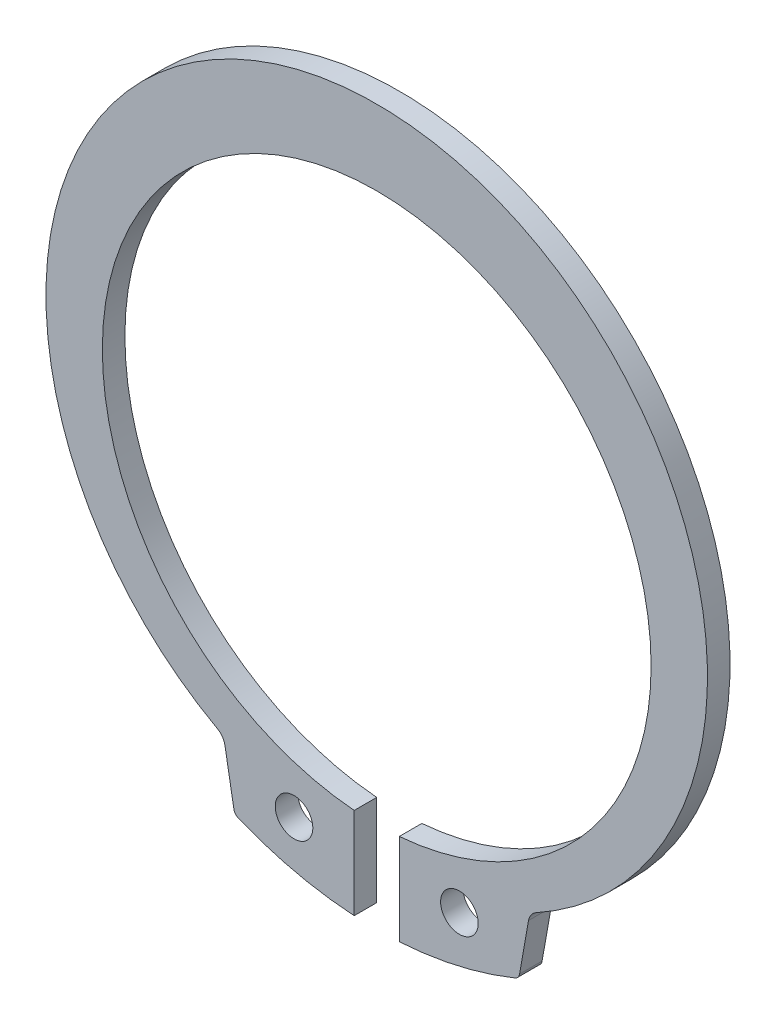
from build123d import *

# Parameters (mm, degrees)
EXTRUDE_972_DEPTH      = 0.75
EXTRUDE_972_DEPTH_BACK = 0.75
SKETCH_1_R             = 1.25


with BuildPart() as part:
    # 草图1 → Extrude 972 (new, two sides: drawn at the far end of the back side and taken through both)
    with BuildSketch(Plane.XY.offset(-EXTRUDE_972_DEPTH_BACK)):
        with BuildLine():
            Line((-1.5, -19.438251703), (-1.5, -25.503659518))
            ThreePointArc((-1.5, -25.503659518), (-5.420429348, -24.937738298), (-9.196831336, -23.742405238))
            ThreePointArc((-9.196831336, -23.742405238), (-9.396824452, -23.593447727), (-9.5, -23.366422634))
            Line((-9.5, -23.366422634), (-10.097014043, -19.980587746))
            ThreePointArc((-10.097014043, -19.980587746), (-10.268699557, -19.572142955), (-10.600003457, -19.277964797))
            ThreePointArc((-10.600003457, -19.277964797), (0, 22), (10.600003457, -19.277964797))
            ThreePointArc((10.600003457, -19.277964797), (10.268699557, -19.572142955), (10.097014043, -19.980587746))
            Line((10.097014043, -19.980587746), (9.5, -23.366422634))
            ThreePointArc((9.5, -23.366422634), (9.396824452, -23.593447727), (9.196831336, -23.742405238))
            ThreePointArc((9.196831336, -23.742405238), (5.420429348, -24.937738298), (1.5, -25.503659518))
            Line((1.5, -25.503659518), (1.5, -19.438251703))
            ThreePointArc((1.5, -19.438251703), (0, 17), (-1.5, -19.438251703))
        make_face()
        with Locations((-5.5, -21.827657787)):
            Circle(SKETCH_1_R, mode=Mode.SUBTRACT)
        with Locations(Location((5.5, -21.827657787, 0), (0, 0, 180))):
            Circle(SKETCH_1_R, mode=Mode.SUBTRACT)
    extrude(amount=EXTRUDE_972_DEPTH + EXTRUDE_972_DEPTH_BACK)


solid = part.part
